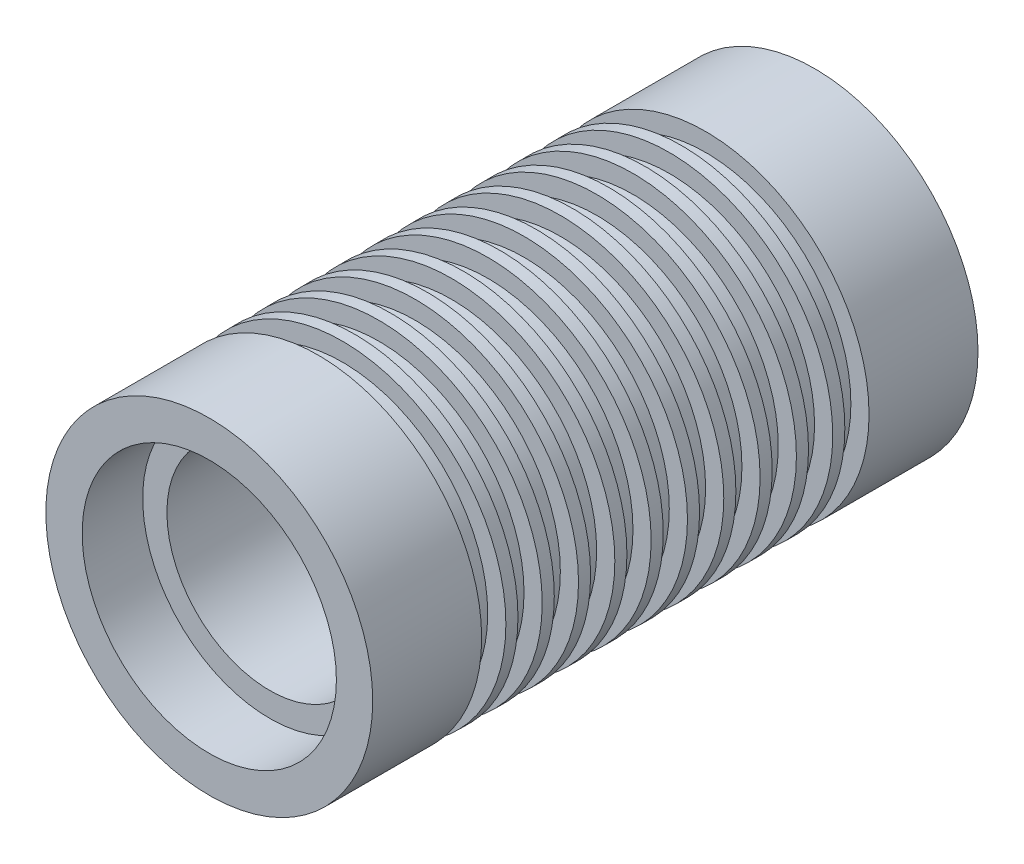
SolidWorks part; units mm, degrees
ref_plane "前视基准面" through (0, 0, 0) normal (0, 0, 1) x (1, 0, 0)
ref_plane "上视基准面" through (0, 0, 0) normal (0, 1, 0) x (1, 0, 0)
ref_plane "右视基准面" through (0, 0, 0) normal (1, 0, 0) x (0, 0, -1)
sketch "草图1" plane through (0, 0, 0) normal (0, 0, 1) x (1, 0, 0)
  circle A0 centre (0, 0) radius 8.5
  circle A1 centre (0, 0) radius 13.5
  dimension "D1" = 17
  dimension "D2" = 27
extrude "凸台-拉伸1" add sketch "草图1" along normal mid plane 50
sketch "草图2" plane through (0, 0, 0) normal (0, 1, 0) x (1, 0, 0)
  line L0 (13.5, 1) -> (12, 1)
  line L1 (13.5, -25) -> (13.5, 25) construction
  line L2 (12, 1) -> (12, -1)
  line L3 (12, -1) -> (13.5, -1)
  line L4 (13.5, -1) -> (13.5, 1)
  line L5 (0, 0) -> (12, 0) construction
  line L6 (0, 0) -> (0, 25) construction
  line L7 (8.5, 25) -> (-8.5, 25) construction
  dimension "D1" = 2
  dimension "D2" = 12
revolve "切除-旋转1" cut sketch "草图2" angle 360 about L6
pattern_linear "阵列(线性)1" count 6 spacing 3 along (0, 0, -1) of "切除-旋转1"
mirror "镜向1" about plane through (0, 0, 0) normal (0, 0, 1) of "阵列(线性)1"
sketch "草图3" plane through (0, 0, 25) normal (0, 0, 1) x (1, 0, 0)
  circle A0 centre (0, 0) radius 10.5
  dimension "D1" = 21
extrude "切除-拉伸1" cut sketch "草图3" against normal blind 5
mirror "镜向2" about plane through (0, 0, 0) normal (0, 0, 1) of "切除-拉伸1"
